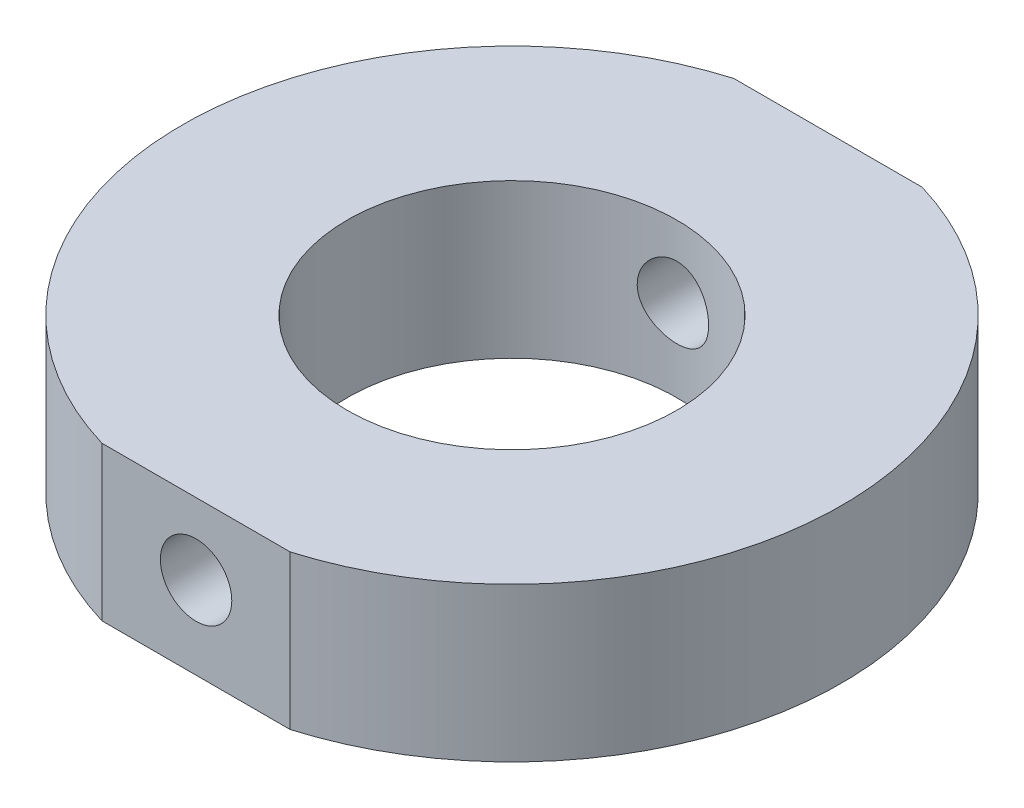
SolidWorks part; units mm, degrees
material "Q235A"
ref_plane "Front Plane" through (0, 0, 0) normal (0, 0, 1) x (1, 0, 0)
ref_plane "Top Plane" through (0, 0, 0) normal (0, 1, 0) x (1, 0, 0)
ref_plane "Right Plane" through (0, 0, 0) normal (1, 0, 0) x (0, 0, -1)
sketch "Sketch1" plane through (0, 0, 0) normal (0, 1, 0) x (1, 0, 0)
  circle A0 centre (0, 0) radius 30
  circle A1 centre (0, 0) radius 60
  dimension "D1" = 120
  dimension "D2" = 60
extrude "Boss-Extrude1" add sketch "Sketch1" along normal mid plane 28
sketch "Sketch2" plane through (0, 0, 0) normal (0, 1, 0) x (1, 0, 0)
  line L0 (0, 0) -> (0, 73.6466) construction
  line L1 (-80, 57.5) -> (80, 57.5)
  line L2 (-80, 57.5) -> (-80, -57.5)
  line L3 (-80, -57.5) -> (80, -57.5)
  line L4 (80, 57.5) -> (80, -57.5)
  line L6 (0, 0) -> (94.7046, 0) construction
  dimension "D1" = 115
  dimension "D2" = 160
extrude "Cut-Extrude1" cut sketch "Sketch2" against normal through all both and the other way through all flip side to cut
sketch "Sketch3" plane through (0, 0, 57.5) normal (0, 0, 1) x (1, 0, 0)
  line L0 (0, 35.1687) -> (0, -33.2063) construction
  line L1 (-17.1391, -14) -> (17.1391, -14) construction
  line L2 (-36.1534, 1) -> (26.3062, 1) construction
  line L3 (-17.1391, -14) -> (17.1391, -14) construction
  circle A0 centre (0, 1) radius 6.5
  dimension "D2" = 13
  dimension "D1" = 15
extrude "Cut-Extrude2" cut sketch "Sketch3" against normal through all
